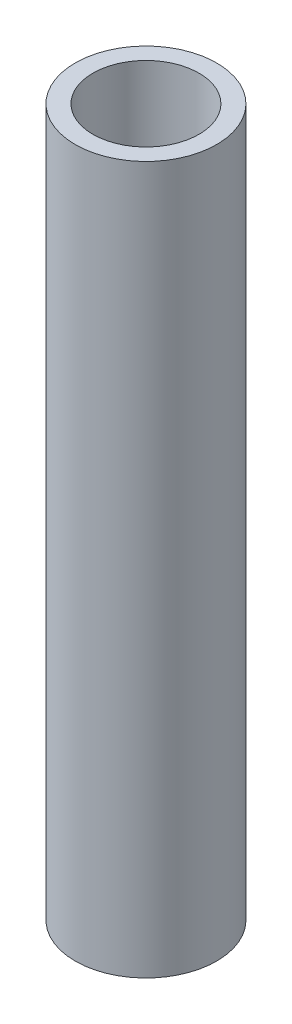
SolidWorks part; units mm, degrees
ref_plane "Front Plane" through (0, 0, 0) normal (0, 0, 1) x (1, 0, 0)
ref_plane "Top Plane" through (0, 0, 0) normal (0, 1, 0) x (1, 0, 0)
ref_plane "Right Plane" through (0, 0, 0) normal (1, 0, 0) x (0, 0, -1)
other "Configuration Table"
sketch "Sketch1" plane through (0, 0, 0) normal (0, 1, 0) x (1, 0, 0)
  circle A0 centre (0, 0) radius 4
  circle A1 centre (0, 0) radius 3
  dimension "D1" = 8
  dimension "D2" = 6
extrude "Boss-Extrude1" add sketch "Sketch1" along normal blind 40
